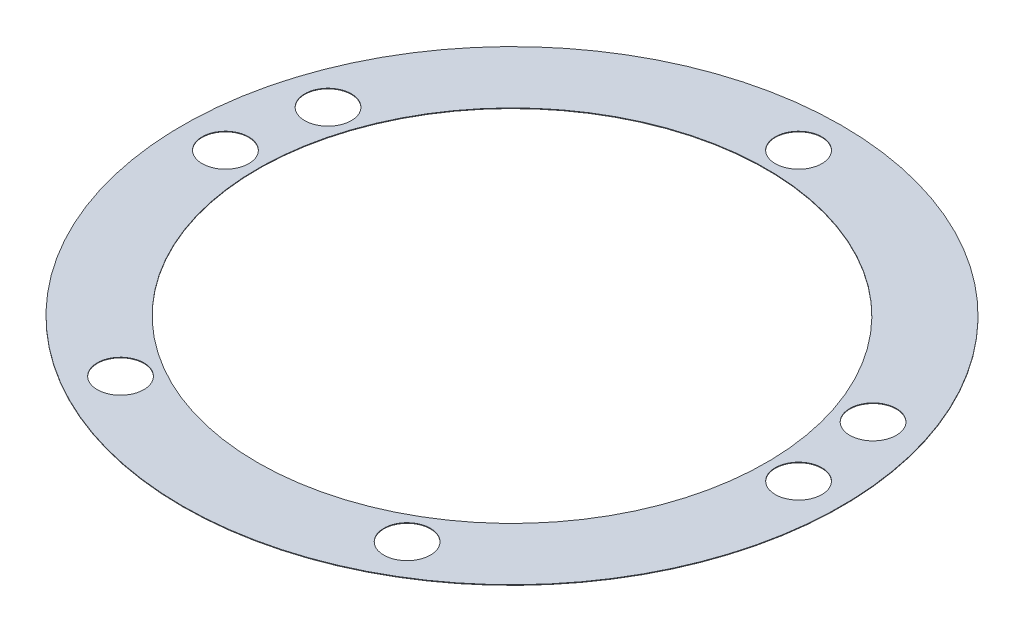
SolidWorks part; units mm, degrees
material "瓦楞纸"
ref_plane "Front Plane" through (0, 0, 0) normal (0, 0, 1) x (1, 0, 0)
ref_plane "Top Plane" through (0, 0, 0) normal (0, 1, 0) x (1, 0, 0)
ref_plane "Right Plane" through (0, 0, 0) normal (1, 0, 0) x (0, 0, -1)
sketch "Sketch1" plane through (0, 0, 0) normal (0, 1, 0) x (1, 0, 0)
  circle A0 centre (0, 0) radius 146.05
  circle A1 centre (0, 0) radius 112.776
  dimension "D1" = 292.1
  dimension "D2" = 225.552
extrude "Boss-Extrude1" add sketch "Sketch1" along normal blind 0.254
hole_wizard "13/16 (0.8125) Diameter Hole1" positions "Sketch3" profile "Sketch2" hole size "13/16" standard "Ansi Inch" end condition through all
sketch "Sketch3" plane through (0, 0.254, 0) normal (0, 1, 0) x (1, 0, 0)
  line L0 (0, -0.1397) -> (0, 0.1397) construction
  line L1 (-0.1397, 0) -> (0.1397, 0) construction
  point P0 (0, 127)
  dimension "D1" = 0
  dimension "D2" = 127
sketch "Sketch2" plane through (0, 0.254, -127) normal (1, 0, 0) x (0, 0, 1)
  line L0 (0, 0) -> (0, 0.254)
  line L1 (0, 0.254) -> (10.3187, 0.254)
  line L2 (10.3187, 0.254) -> (10.3187, 0)
  line L5 (10.3187, 0) -> (0, 0)
  line L11 (0, -6.35) -> (0, 107.95) construction
  dimension "通孔孔直径" = 20.6375
  dimension "通孔孔深度" = 0.254
hole_wizard "13/16 (0.8125) Diameter Hole2" positions "Sketch5" profile "Sketch4" hole size "13/16" standard "Ansi Inch" end condition through all
sketch "Sketch5" plane through (0, 0, 0) normal (0, -1, 0) x (-1, 0, 0)
  line L0 (-0.1397, 0) -> (0.1397, 0) construction
  line L1 (0, 0.1397) -> (0, -0.1397) construction
  point P0 (-63.5, -109.982)
  point P2 (-120.77, 39.243)
  point P9 (-127, 0)
  dimension "D1" = 109.982
  dimension "D2" = 63.5
  dimension "D3" = 39.243
  dimension "D4" = 120.77
  dimension "D5" = 0
  dimension "D6" = 127
sketch "Sketch4" plane through (63.5, 0, 109.982) normal (1, 0, 0) x (0, 0, -1)
  line L0 (0, 0) -> (0, 0.254)
  line L1 (0, 0.254) -> (10.3187, 0.254)
  line L2 (10.3187, 0.254) -> (10.3187, 0)
  line L5 (10.3187, 0) -> (0, 0)
  line L11 (0, -6.35) -> (0, 107.95) construction
  dimension "通孔孔直径" = 20.6375
  dimension "通孔孔深度" = 0.254
mirror "Mirror1" about plane through (0, 0, 0) normal (1, 0, 0) of "13/16 (0.8125) Diameter Hole2"
